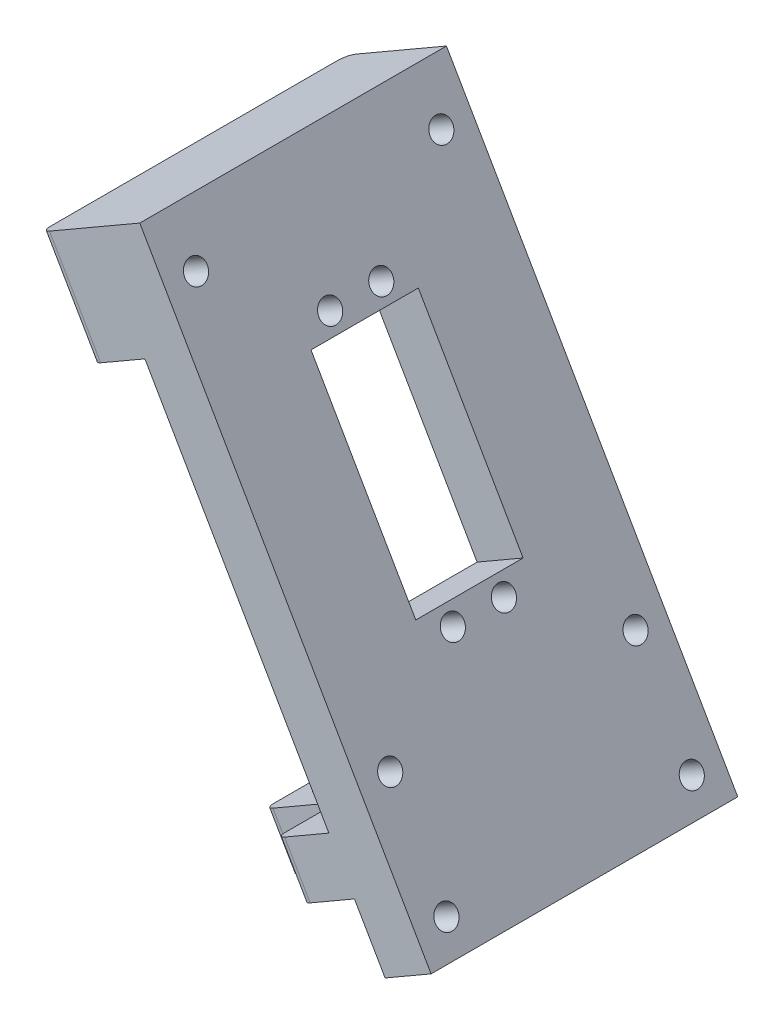
SolidWorks part; units mm, degrees
ref_plane "前视基准面" through (0, 0, 0) normal (0, 0, 1) x (1, 0, 0)
ref_plane "上视基准面" through (0, 0, 0) normal (0, 1, 0) x (1, 0, 0)
ref_plane "右视基准面" through (0, 0, 0) normal (1, 0, 0) x (0, 0, -1)
sketch "草图1" plane through (0, 0, 0) normal (0, 0, 1) x (1, 0, 0)
  line L1 (6, -13) -> (-6, -13)
  line L2 (6, -13) -> (6, 13)
  line L3 (6, 13) -> (-6, 13)
  line L4 (-6, -13) -> (-6, 13)
  line L5 (6, -13) -> (-6, 13) construction
  line L6 (6, 13) -> (-6, -13) construction
  point P0 (0, 0)
  dimension "D1" = 26
  dimension "D2" = 12
extrude "凸台-拉伸1" add sketch "草图1" along normal mid plane 60 contours L3 L4 L1 L2
sketch "草图2" plane through (0, 0, -30) normal (0, 0, -1) x (-1, 0, 0)
  line L0 (6, 13) -> (71, 125.5833)
  line L1 (71, 125.5833) -> (62, 130.7795)
  line L2 (62, 130.7795) -> (-6, 13)
  line L3 (-6, 13) -> (6, 13) construction
  line L4 (-6, 13) -> (6, 13)
  line L5 (6, -13) -> (6, 13) construction
  line L6 (-6, -13) -> (-6, 13) construction
  dimension "D1" = 150
  dimension "D2" = 130
extrude "凸台-拉伸2" add sketch "草图2" against normal up to surface (60 mm away) up to face at (0, 0, 30)
sketch "草图3" plane through (1.1292, 0.6519, 0) normal (-0.866, -0.5, 0) x (0, 0, 1)
  line L0 (30, 14.2583) -> (30, 144.2583) construction
  line L1 (-30, 144.2583) -> (30, 144.2583)
  line L2 (-30, 144.2583) -> (-30, 124.2583)
  line L3 (-30, 124.2583) -> (30, 124.2583)
  line L4 (30, 144.2583) -> (30, 124.2583)
  line L5 (-30, 144.2583) -> (30, 124.2583) construction
  line L6 (-30, 124.2583) -> (30, 144.2583) construction
  point P0 (0, 134.2583)
  dimension "D1" = 20
extrude "凸台-拉伸3" add sketch "草图3" along normal blind 12
sketch "草图5" plane through (-62.1292, 107.6109, 0) normal (0.5, -0.866, 0) x (0, 0, -1)
  line L10 (30, 1.3038) -> (-30, 1.3038) construction
  line L11 (30, 1.3038) -> (-30, 1.3038)
  line L16 (30, -10.6962) -> (-30, -10.6962) construction
  line L21 (30, -10.6962) -> (-30, -10.6962)
  line L22 (-13, -10.6962) -> (-13, -22.1962)
  line L23 (-13, -22.1962) -> (13, -22.1962)
  line L24 (13, -22.1962) -> (13, -10.6962)
  line L25 (0, -10.6962) -> (0, -22.1962) construction
  line L26 (-18, -10.6962) -> (-18, -27.1962)
  line L27 (-18, -27.1962) -> (18, -27.1962)
  line L28 (18, -27.1962) -> (18, -10.6962)
  line L29 (-30, 1.3038) -> (-30, -10.6962)
  line L30 (30, 1.3038) -> (30, -10.6962)
  dimension "D1" = 11.5
  dimension "D2" = 26
  dimension "D3" = 5
extrude "凸台-拉伸4" add sketch "草图5" along normal blind 10 from offset 72
sketch "草图6" plane through (10.1292, 5.8481, 0) normal (0.866, 0.5, 0) x (0, 0, -1)
  line L0 (-30, 144.2583) -> (30, 144.2583) construction
  line L1 (10.5, 75.2583) -> (-10.5, 75.2583)
  line L2 (10.5, 75.2583) -> (10.5, 116.2583)
  line L3 (10.5, 116.2583) -> (-10.5, 116.2583)
  line L4 (-10.5, 75.2583) -> (-10.5, 116.2583)
  line L5 (10.5, 75.2583) -> (-10.5, 116.2583) construction
  line L6 (10.5, 116.2583) -> (-10.5, 75.2583) construction
  line L7 (0, 95.7583) -> (0, 144.2583) construction
  point P0 (0, 95.7583)
  dimension "D1" = 21
  dimension "D2" = 41
  dimension "D3" = 28
extrude "切除-拉伸1" cut sketch "草图6" against normal blind 55
sketch "草图7" plane through (10.1292, 5.8481, 0) normal (0.866, 0.5, 0) x (0, 0, -1)
  line L0 (5, 119.7583) -> (5, 71.7583) construction
  line L1 (-5, 119.7583) -> (5, 119.7583) construction
  line L2 (-5, 119.7583) -> (5, 71.7583) construction
  line L3 (10.5, 95.7583) -> (5, 95.7583) construction
  line L4 (10.5, 75.2583) -> (10.5, 116.2583) construction
  line L5 (5, 71.7583) -> (-5, 71.7583) construction
  line L6 (-5, 71.7583) -> (-5, 119.7583) construction
  line L7 (0, 95.7583) -> (0, 75.2583) construction
  line L8 (-10.5, 75.2583) -> (10.5, 75.2583) construction
  circle A4 centre (5, 71.7583) radius 2.2
  circle A5 centre (-5, 71.7583) radius 2.2
  circle A6 centre (5, 119.7583) radius 2.2
  circle A7 centre (-5, 119.7583) radius 2.2
  dimension "D3" = 4.4
  dimension "D1" = 10
  dimension "D2" = 48
extrude "切除-拉伸2" cut sketch "草图7" against normal blind 41
fillet "圆角1" radius 20 2 edges at (-6, 13, 0) (6, 13, 0)
sketch "草图8" plane through (-6, 0, 0) normal (-1, 0, 0) x (0, 0, 1)
  line L0 (30, -13) -> (-30, -13) construction
  line L1 (12.5, -3) -> (-12.5, -3) construction
  line L2 (12.5, -3) -> (12.5, -13) construction
  line L3 (12.5, -13) -> (-12.5, -13) construction
  line L4 (-12.5, -3) -> (-12.5, -13) construction
  line L5 (12.5, -3) -> (-12.5, -13) construction
  line L6 (12.5, -13) -> (-12.5, -3) construction
  line L7 (0, -8) -> (0, 0) construction
  circle A0 centre (-12.5, -3) radius 3.3
  circle A1 centre (12.5, -3) radius 3.3
  point P0 (0, -8)
  dimension "D3" = 6.6
  dimension "D1" = 10
  dimension "D2" = 25
extrude "切除-拉伸3" cut sketch "草图8" against normal blind 21
fillet "圆角2" radius 2 2 edges at (0, -13, -30) (0, -13, 30)
fillet "圆角3" radius 2 6 edges at (-32.8923, 35.5788, -30) (-32.8923, 35.5788, 30) (-32.8923, 35.5788, 18) (-47.1817, 27.3288, 18) (-47.1817, 27.3288, -18) (-32.8923, 35.5788, -18)
fillet "圆角4" radius 2 2 edges at (-76.3923, 110.923, -30) (-76.3923, 110.923, 30)
sketch "草图9" plane through (1.1292, 0.6519, 0) normal (-0.866, -0.5, 0) x (0, 0, 1)
  line L0 (-30, 19.6173) -> (-30, 42.2583) construction
  line L1 (30, -30.2583) -> (-30, -30.2583)
  line L2 (30, -30.2583) -> (30, 30.2583)
  line L3 (30, 30.2583) -> (-30, 30.2583)
  line L4 (-30, -30.2583) -> (-30, 30.2583)
  line L5 (30, -30.2583) -> (-30, 30.2583) construction
  line L6 (30, 30.2583) -> (-30, -30.2583) construction
  line L7 (16, 42.2583) -> (-16, 42.2583) construction
  point P0 (0, 0)
  dimension "D1" = 12
extrude "切除-拉伸4" cut sketch "草图9" against normal mid plane 70
sketch "草图10" plane through (-9.2631, -5.3481, 0) normal (-0.866, -0.5, 0) x (0, 0, 1)
  line L0 (-30, 134.2583) -> (-24, 134.2583) construction
  line L1 (-30, 124.2583) -> (-30, 144.2583) construction
  line L2 (-24, 134.2583) -> (24, 134.2583) construction
  line L3 (24, 134.2583) -> (30, 134.2583) construction
  line L4 (30, 144.2583) -> (30, 124.2583) construction
  circle A0 centre (24, 134.2583) radius 2.2
  circle A1 centre (-24, 134.2583) radius 2.2
  dimension "D2" = 4.4
  dimension "D1" = 48
extrude "切除-拉伸5" cut sketch "草图10" against normal blind 71
sketch "草图12" plane through (1.1292, 0.6519, 0) normal (-0.866, -0.5, 0) x (0, 0, 1)
  line L0 (-28, 47.2583) -> (28, 47.2583) construction
  line L1 (-28, 52.2583) -> (-28, 42.2583) construction
  line L2 (28, 42.2583) -> (28, 52.2583) construction
  line L3 (-30, 42.2583) -> (30, 42.2583) construction
  line L4 (24, 36.2583) -> (-24, 36.2583) construction
  line L5 (24, 36.2583) -> (24, 58.2583) construction
  line L6 (24, 58.2583) -> (-24, 58.2583) construction
  line L7 (-24, 36.2583) -> (-24, 58.2583) construction
  line L8 (24, 36.2583) -> (-24, 58.2583) construction
  line L9 (24, 58.2583) -> (-24, 36.2583) construction
  line L10 (30, 52.2583) -> (30, 124.2583) construction
  circle A0 centre (-24, 58.2583) radius 2.2
  circle A1 centre (24, 58.2583) radius 2.2
  circle A2 centre (24, 36.2583) radius 2.2
  circle A3 centre (-24, 36.2583) radius 2.2
  point P6 (0, 47.2583)
  dimension "D3" = 4.4
  dimension "D1" = 6
  dimension "D2" = 6
extrude "切除-拉伸6" cut sketch "草图12" against normal blind 113
